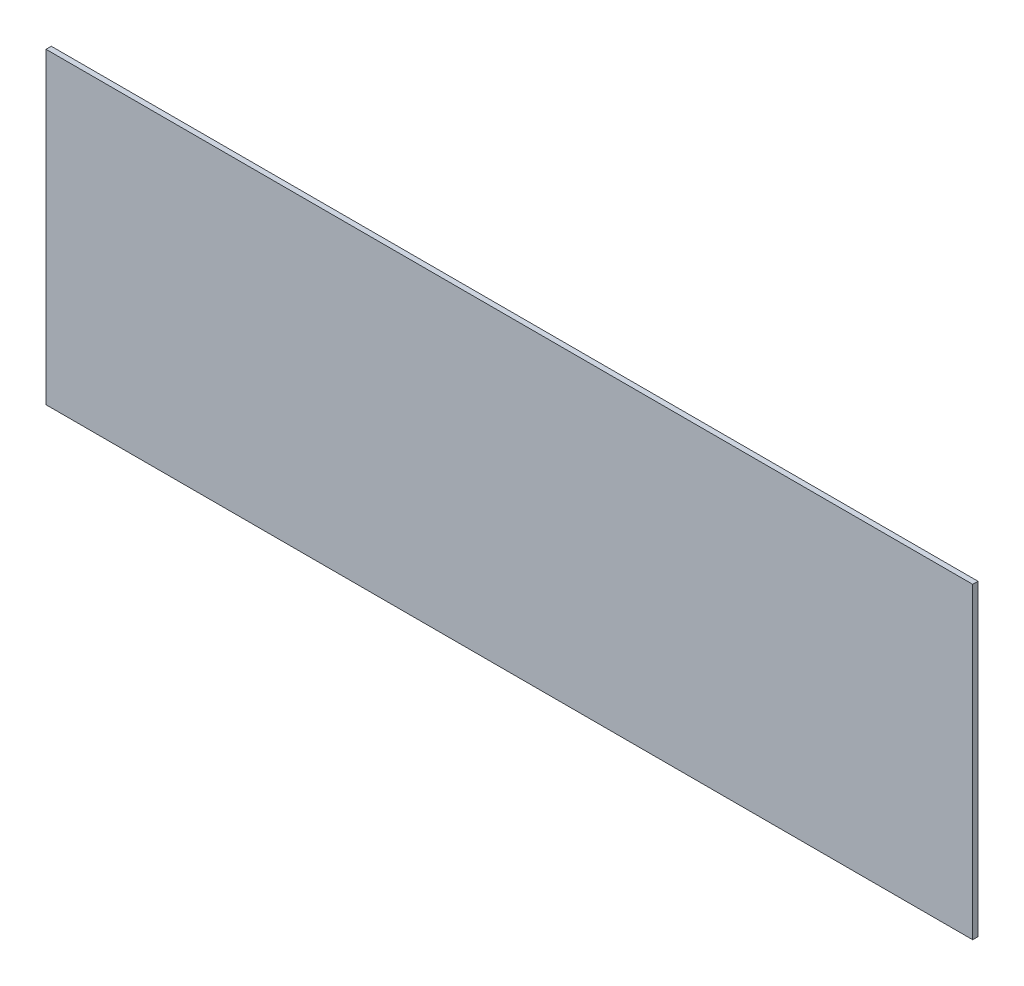
from build123d import *

# Parameters (mm, degrees)
SKETCH_1_W      = 876
SKETCH_1_H      = 291
EXTRUDE_1_DEPTH = 5


with BuildPart() as part:
    # 草图1 → 凸台-拉伸1 (new body)
    with BuildSketch(Plane.XY):
        Rectangle(SKETCH_1_W, SKETCH_1_H)
    extrude(amount=EXTRUDE_1_DEPTH)


solid = part.part
